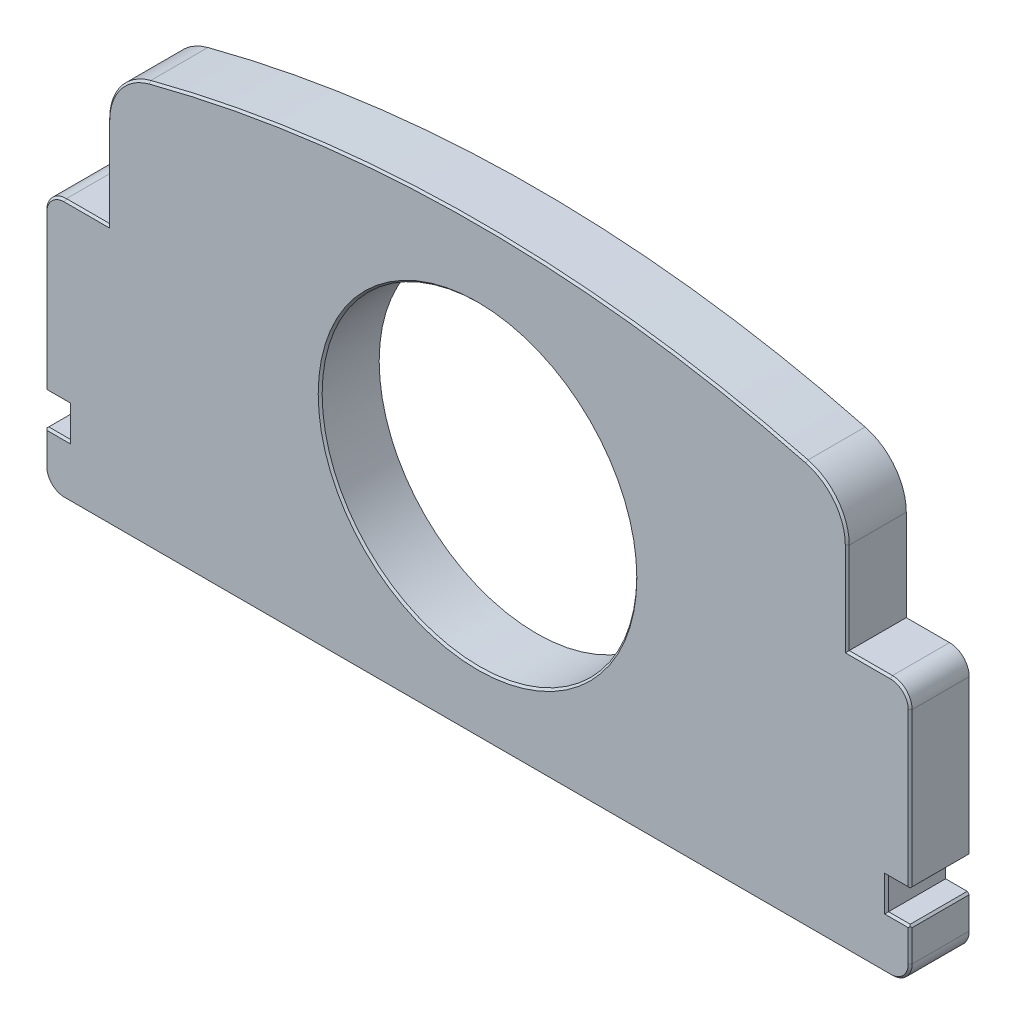
from build123d import *

# Parameters (mm, degrees)
SKETCH_1_W           = 220
SKETCH_1_H           = 121
EXTRUDE_1_DEPTH      = 7.5
SKETCH_5_W           = 6
SKETCH_5_H           = 8
CUT_EXTRUDE_2_DEPTH  = 165.213275955
SKETCH_9_R           = 22.5
CUT_EXTRUDE_5_DEPTH  = 10
CUT_EXTRUDE_12_DEPTH = 165.213275955
FILLET_1_R           = 5
CHAMFER_1_SIZE       = 0.5
SKETCH_19_R          = 40
CUT_EXTRUDE_13_DEPTH = 159.767912375
CHAMFER_2_SIZE       = 0.5
CHAMFER_4_SIZE       = 0.5


with BuildPart() as part:
    # 草图1 → 凸台-拉伸1 (new, symmetric)
    with BuildSketch(Plane.XY):
        with Locations((0, 60.5)):
            Rectangle(SKETCH_1_W, SKETCH_1_H)
    extrude(amount=EXTRUDE_1_DEPTH, both=True)

    # 草图5 → 切除-拉伸2 (cut, through all)
    with BuildSketch(Plane.XY.offset(7.5)):
        with Locations((-107, 17.5)):
            Rectangle(SKETCH_5_W, SKETCH_5_H)
        with Locations((107, 17.5)):
            Rectangle(SKETCH_5_W, SKETCH_5_H)
    extrude(amount=-CUT_EXTRUDE_2_DEPTH, mode=Mode.SUBTRACT)

    # 草图9 → 切除-拉伸5 (cut)
    with BuildSketch(Plane(origin=(0, 0, -7.5), x_dir=(-1, 0, 0), z_dir=(0, 0, -1))):
        with Locations((0, 66.5)):
            Circle(SKETCH_9_R)
    extrude(amount=-CUT_EXTRUDE_5_DEPTH, mode=Mode.SUBTRACT)

    # 草图4 → 切除-拉伸12 (cut, through all)
    with BuildSketch(Plane.XY.offset(7.5)):
        with BuildLine():
            Line((-94, 66), (-110, 66))
            Line((-110, 66), (-110, 122.2))
            Line((-110, 122.2), (110, 122.2))
            Line((110, 122.2), (110, 66))
            Line((110, 66), (94, 66))
            Line((94, 66), (94, 89.205740869))
            ThreePointArc((94, 89.205740869), (91.081973046, 97.760848899), (83.544303797, 102.749666097))
            ThreePointArc((83.544303797, 102.749666097), (0, 113.5), (-83.544303797, 102.749666097))
            ThreePointArc((-83.544303797, 102.749666097), (-91.081973046, 97.760848899), (-94, 89.205740869))
            Line((-94, 89.205740869), (-94, 66))
        make_face()
    extrude(amount=-CUT_EXTRUDE_12_DEPTH, mode=Mode.SUBTRACT)

    # 圆角1
    fillet_1_edges = [part.edges().sort_by_distance(p)[0] for p in [
        (-110, 66, 0),
        (110, 66, 0),
        (110, 0, 0),
        (-110, 0, 0),
    ]]
    fillet(fillet_1_edges, radius=FILLET_1_R)

    # 倒角1
    chamfer_1_edges = [part.edges().sort_by_distance(p)[0] for p in [
        (-110, 9.25, 7.5),
        (-107, 13.5, 7.5),
        (-104, 17.5, 7.5),
        (-107, 21.5, 7.5),
        (110, 41.25, 7.5),
        (107, 21.5, 7.5),
        (104, 17.5, 7.5),
        (107, 13.5, 7.5),
        (-94, 77.602870434, 7.5),
        (-91.081973046, 97.760848899, 7.5),
        (0, 113.5, 7.5),
        (91.081973046, 97.760848899, 7.5),
        (94, 77.602870434, 7.5),
        (99.5, 66, 7.5),
        (110, 9.25, 7.5),
        (0, 0, 7.5),
        (-99.5, 66, 7.5),
        (-110, 41.25, 7.5),
        (-108.535533906, 64.535533906, 7.5),
        (108.535533906, 64.535533906, 7.5),
        (-108.535533906, 1.464466094, 7.5),
        (108.535533906, 1.464466094, 7.5),
    ]]
    chamfer(chamfer_1_edges, length=CHAMFER_1_SIZE)

    # 草图19 → 切除-拉伸13 (cut, through all)
    with BuildSketch(Plane.XY.offset(7.5)):
        with Locations((0, 55.5)):
            Circle(SKETCH_19_R)
    extrude(amount=-CUT_EXTRUDE_13_DEPTH, mode=Mode.SUBTRACT)

    # 倒角2
    chamfer_2_edges = [part.edges().sort_by_distance(p)[0] for p in [
        (-40, 55.5, 7.5),
    ]]
    chamfer(chamfer_2_edges, length=CHAMFER_2_SIZE)

    # 倒角4
    chamfer_4_edges = [part.edges().sort_by_distance(p)[0] for p in [
        (-110, 13.5, -0.25),
        (-110, 21.5, -0.25),
        (110, 21.5, -0.25),
        (110, 13.5, -0.25),
    ]]
    chamfer(chamfer_4_edges, length=CHAMFER_4_SIZE)


solid = part.part
